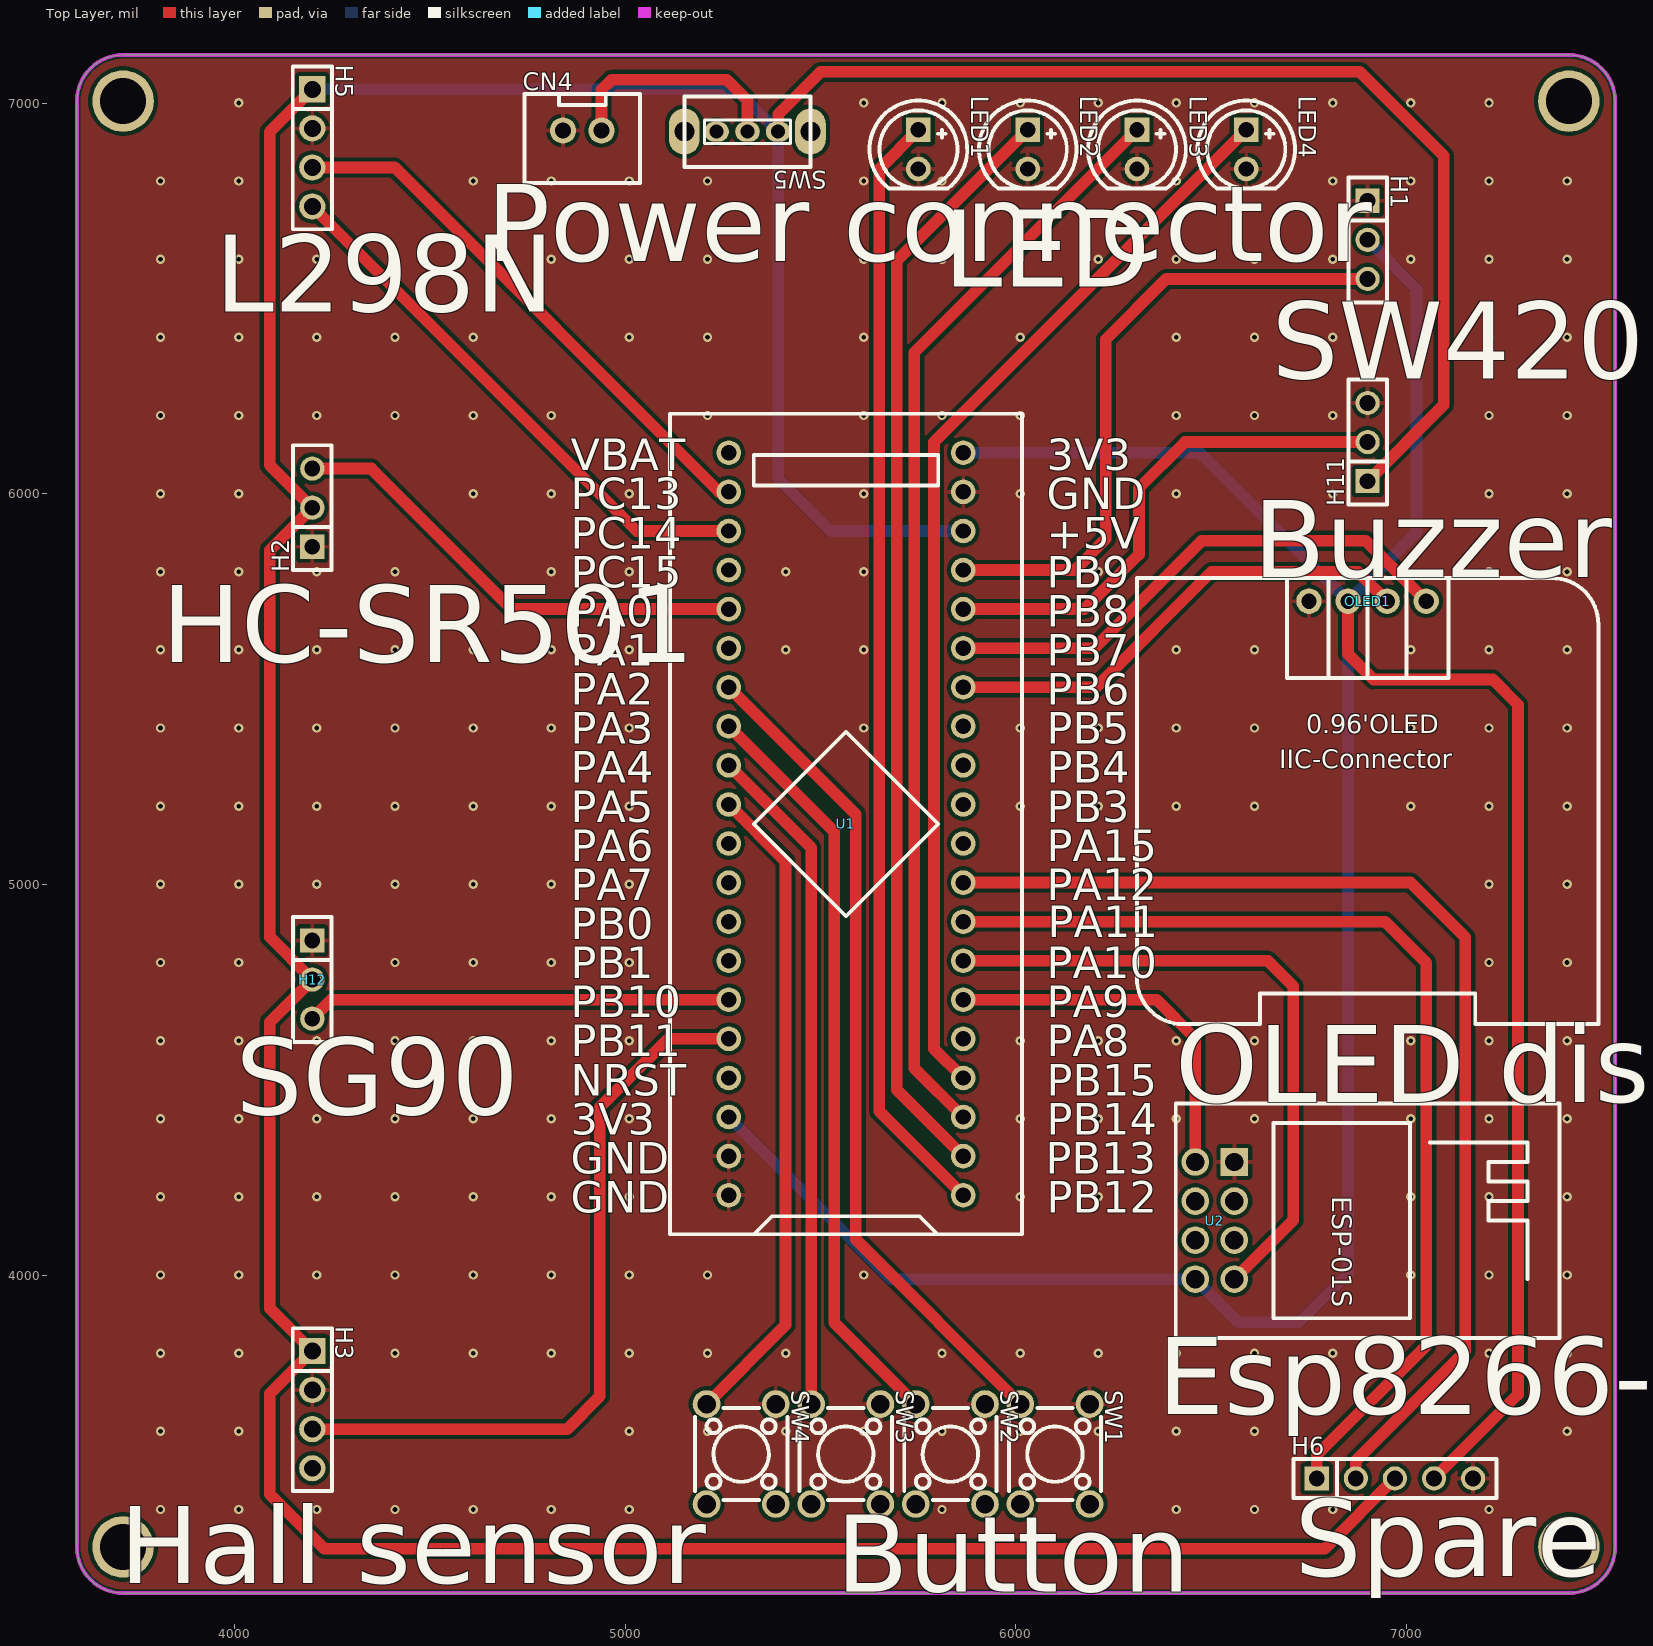
[diagram p0: Top Layer view]
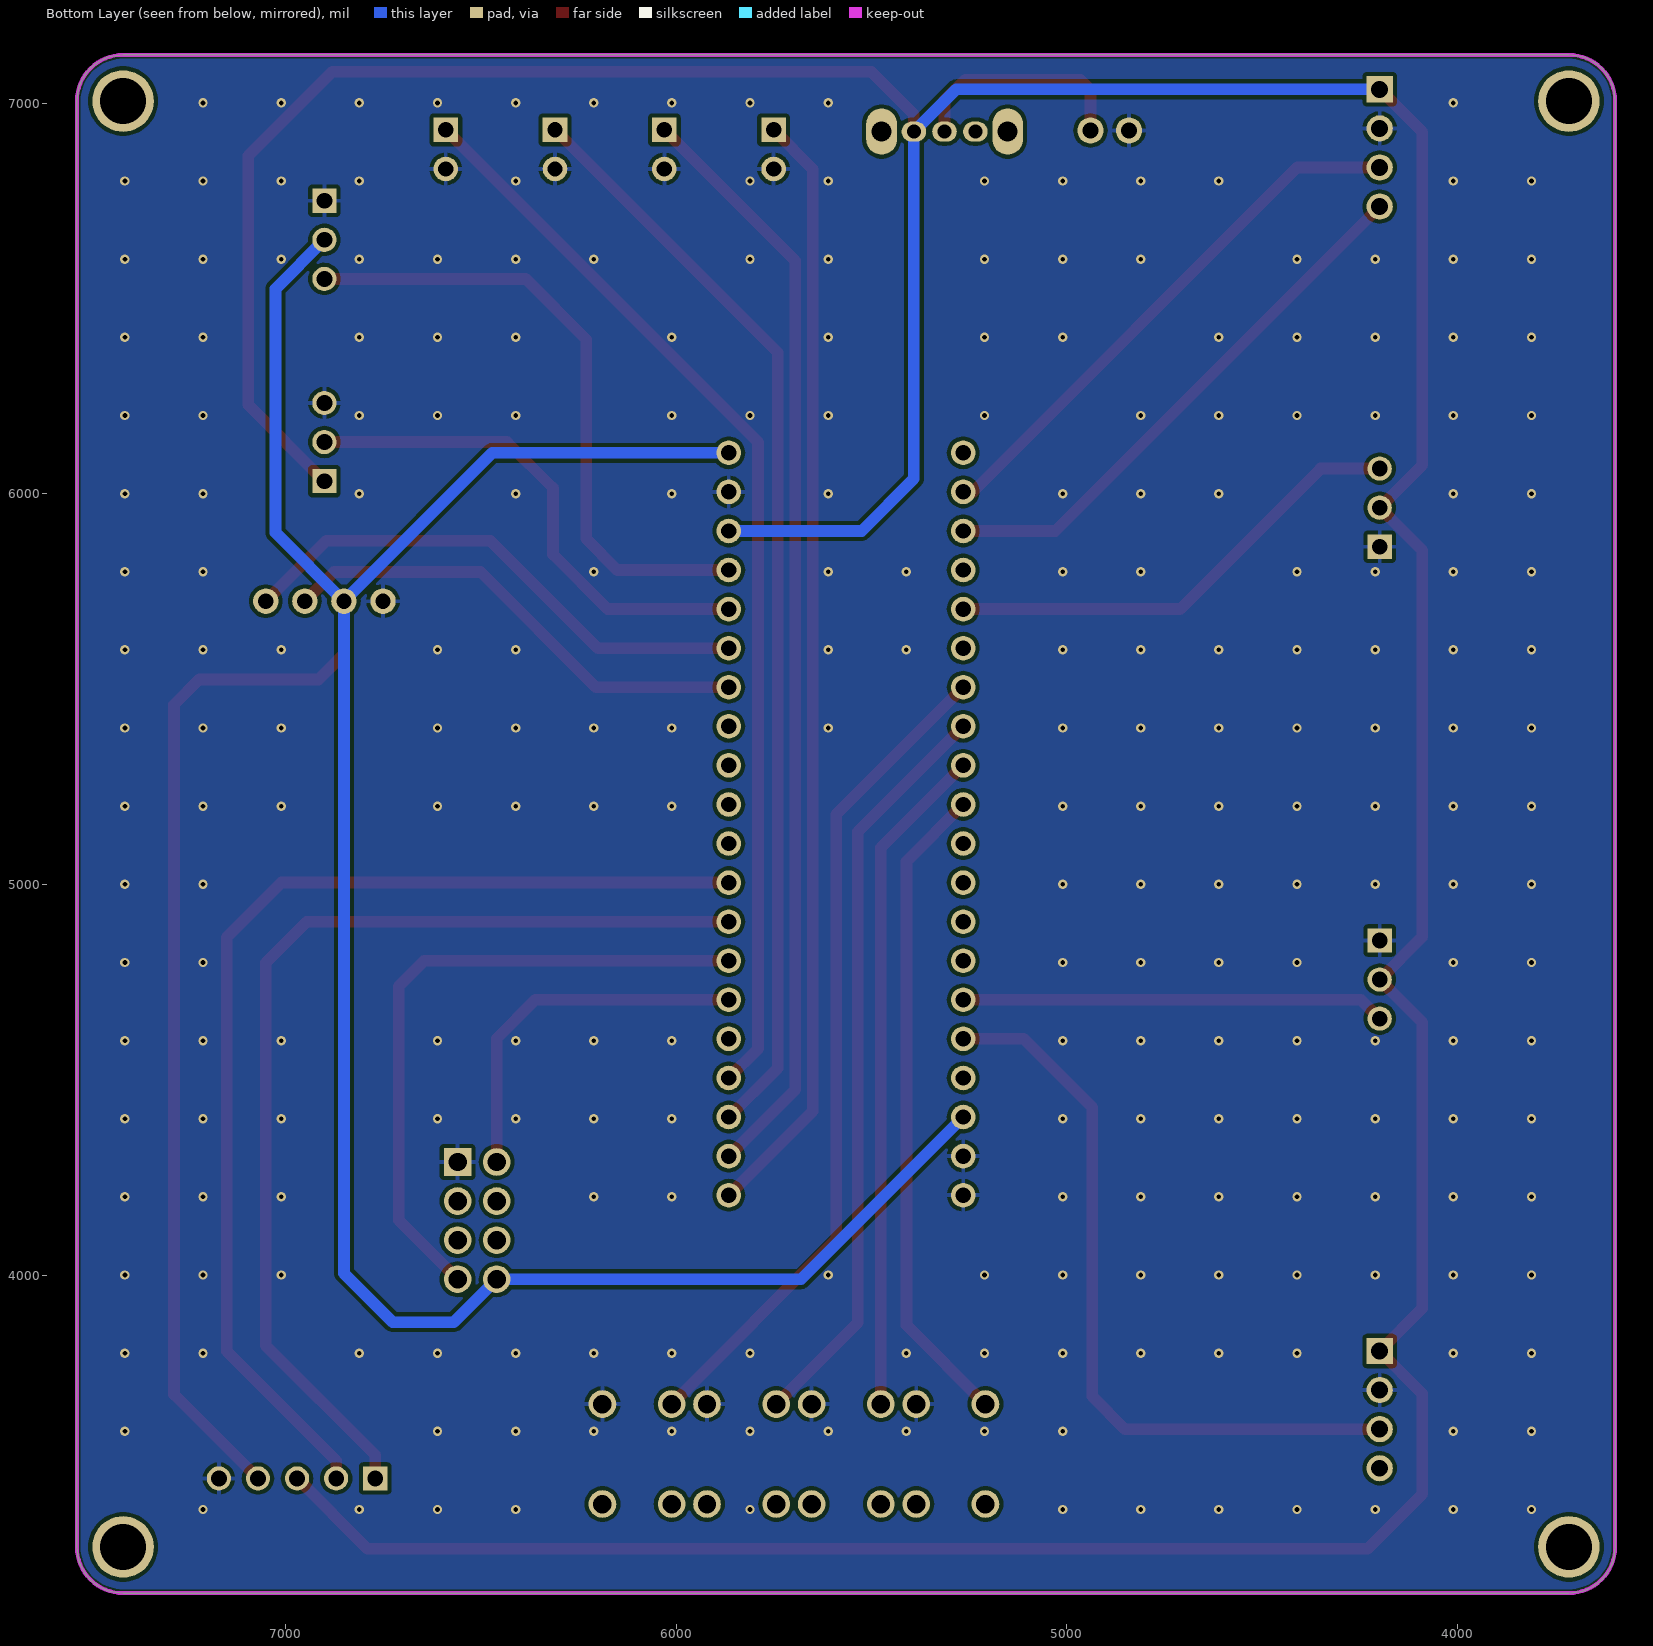
[diagram p1: Bottom Layer view, seen from below]
# Altium PCB MISC51767.pcbdoc
Units mil, origin at the board's own origin, x right, y up, seen from the top; angles counter-clockwise.
Board outline 3937.01 x 3937.01 mil, 2 copper layers (Top Layer, Bottom Layer), stack 62.206 mil thick; 20 components, 38 nets, 112 pads, 242 vias.

## Layer stack, top to bottom
Top Solder Mask Layer: solder mask 0.394, Dk 3.3
Top Layer: signal copper 1.379
Dielectric1: surface 59.449, FR4, Dk 4.5
Bottom Layer: signal copper 1.378
Bottom Solder Mask Layer: solder mask 0.394, Dk 3.3

## Board outline
3714.61,7123.5 ccw(c3714.61,7005.39) 3596.5,7005.39 3596.5,3304.61 ccw(c3714.61,3304.61) 3714.61,3186.5 7415.39,3186.5 ccw(c7415.39,3304.61) 7533.5,3304.61 7533.5,7005.39 ccw(c7415.39,7005.39) 7415.39,7123.5 3714.61,7123.5

## Design rules (kind name [scope] priority, off if disabled: settings)
BoardOutlineClearance copperThickness2oz_1 [All] p2 off: genericclearance=7.99 ignorepadtopadclearanceinfootprint=FALSE except(0: Arc-SplitContinuation Track-SplitContinuation SMDPad-SplitContinuation THPad-SplitContinuation Via-SplitContinuation Fill-SplitContinuation Region-SplitContinuation Poly-SplitContinuation Text-SplitContinuation Hole-SplitContinuation; 5.98: Arc-CutoutEdge Track-CutoutEdge SMDPad-CutoutEdge THPad-CutoutEdge Via-CutoutEdge Text-CutoutEdge; 6.9: Hole-OutlineEdge Hole-CutoutEdge; 10: Poly-OutlineEdge Poly-CutoutEdge; 11.81: Arc-OutlineEdge Track-OutlineEdge SMDPad-OutlineEdge THPad-OutlineEdge Via-OutlineEdge Fill-OutlineEdge Region-OutlineEdge Text-OutlineEdge Fill-CutoutEdge Region-CutoutEdge)
BoardOutlineClearance Plane_innerPlane_1 [All] p4 off: genericclearance=4.02 ignorepadtopadclearanceinfootprint=FALSE except(0: Arc-SplitContinuation Track-SplitContinuation SMDPad-SplitContinuation THPad-SplitContinuation Via-SplitContinuation Fill-SplitContinuation Region-SplitContinuation Poly-SplitContinuation Text-SplitContinuation Hole-SplitContinuation; 5.98: Arc-CutoutEdge Track-CutoutEdge SMDPad-CutoutEdge THPad-CutoutEdge Via-CutoutEdge Text-CutoutEdge; 6.9: Hole-OutlineEdge Hole-CutoutEdge; 10: Poly-OutlineEdge Poly-CutoutEdge; 11.81: Arc-OutlineEdge Track-OutlineEdge SMDPad-OutlineEdge THPad-OutlineEdge Via-OutlineEdge Fill-OutlineEdge Region-OutlineEdge Text-OutlineEdge Fill-CutoutEdge Region-CutoutEdge)
BoardOutlineClearance Copper_copperRegion_1 [All] p6 off: genericclearance=4.02 ignorepadtopadclearanceinfootprint=FALSE except(0: Arc-SplitContinuation Track-SplitContinuation SMDPad-SplitContinuation THPad-SplitContinuation Via-SplitContinuation Fill-SplitContinuation Region-SplitContinuation Poly-SplitContinuation Text-SplitContinuation Hole-SplitContinuation; 5.98: Arc-CutoutEdge Track-CutoutEdge SMDPad-CutoutEdge THPad-CutoutEdge Via-CutoutEdge Text-CutoutEdge; 6.9: Hole-OutlineEdge Hole-CutoutEdge; 10: Poly-OutlineEdge Poly-CutoutEdge; 11.81: Arc-OutlineEdge Track-OutlineEdge SMDPad-OutlineEdge THPad-OutlineEdge Via-OutlineEdge Fill-OutlineEdge Region-OutlineEdge Text-OutlineEdge Fill-CutoutEdge Region-CutoutEdge)
BoardOutlineClearance copperThickness1oz_1 [All] p8: genericclearance=4.02 ignorepadtopadclearanceinfootprint=FALSE except(0: Arc-SplitContinuation Track-SplitContinuation SMDPad-SplitContinuation THPad-SplitContinuation Via-SplitContinuation Fill-SplitContinuation Region-SplitContinuation Poly-SplitContinuation Text-SplitContinuation Hole-SplitContinuation; 5.98: Arc-CutoutEdge Track-CutoutEdge SMDPad-CutoutEdge THPad-CutoutEdge Via-CutoutEdge Text-CutoutEdge; 6.9: Hole-OutlineEdge Hole-CutoutEdge; 10: Poly-OutlineEdge Poly-CutoutEdge; 11.81: Arc-OutlineEdge Track-OutlineEdge SMDPad-OutlineEdge THPad-OutlineEdge Via-OutlineEdge Fill-OutlineEdge Region-OutlineEdge Text-OutlineEdge Fill-CutoutEdge Region-CutoutEdge)
Clearance copperThickness2oz [All] p1 off: gap=7.99 ignorepadtopadclearanceinfootprint=FALSE except(5.98: SMDPad-Track SMDPad-SMDPad THPad-Track SMDPad-THPad THPad-THPad Track-Via SMDPad-Via THPad-Via Via-Via Fill-SMDPad Region-SMDPad Fill-THPad Region-THPad Fill-Via Region-Via Fill-Fill Fill-Region Region-Region Arc-Track Arc-SMDPad Arc-THPad Arc-Via Fill-Arc Region-Arc Arc-Arc Text-Track SMDPad-Text Text-THPad Text-Via Fill-Text Region-Text Arc-Text Text-Text; 6.9: Hole-Track Hole-SMDPad Hole-THPad Hole-Via Fill-Hole Region-Hole Hole-Arc Hole-Text; 10: Poly-Track Poly-SMDPad Poly-THPad Poly-Via Poly-Fill Poly-Region Poly-Poly Poly-Arc Poly-Text Poly-Hole; 11.81: Fill-Track Region-Track)
Clearance Plane_innerPlane [All] p3 off: gap=4.02 ignorepadtopadclearanceinfootprint=FALSE except(5.98: SMDPad-Track SMDPad-SMDPad THPad-Track SMDPad-THPad THPad-THPad Track-Via SMDPad-Via THPad-Via Via-Via Fill-SMDPad Region-SMDPad Fill-THPad Region-THPad Fill-Via Region-Via Fill-Fill Fill-Region Region-Region Arc-Track Arc-SMDPad Arc-THPad Arc-Via Fill-Arc Region-Arc Arc-Arc Text-Track SMDPad-Text Text-THPad Text-Via Fill-Text Region-Text Arc-Text Text-Text; 6.9: Hole-Track Hole-SMDPad Hole-THPad Hole-Via Fill-Hole Region-Hole Hole-Arc Hole-Text; 10: Poly-Track Poly-SMDPad Poly-THPad Poly-Via Poly-Fill Poly-Region Poly-Poly Poly-Arc Poly-Text Poly-Hole; 11.81: Fill-Track Region-Track)
Clearance Copper_copperRegion [All] p5 off: gap=4.02 ignorepadtopadclearanceinfootprint=FALSE except(5.98: SMDPad-Track SMDPad-SMDPad THPad-Track SMDPad-THPad THPad-THPad Track-Via SMDPad-Via THPad-Via Via-Via Fill-SMDPad Region-SMDPad Fill-THPad Region-THPad Fill-Via Region-Via Fill-Fill Fill-Region Region-Region Arc-Track Arc-SMDPad Arc-THPad Arc-Via Fill-Arc Region-Arc Arc-Arc Text-Track SMDPad-Text Text-THPad Text-Via Fill-Text Region-Text Arc-Text Text-Text; 6.9: Hole-Track Hole-SMDPad Hole-THPad Hole-Via Fill-Hole Region-Hole Hole-Arc Hole-Text; 10: Poly-Track Poly-SMDPad Poly-THPad Poly-Via Poly-Fill Poly-Region Poly-Poly Poly-Arc Poly-Text Poly-Hole; 11.81: Fill-Track Region-Track)
Clearance copperThickness1oz [All] p7: gap=4.02 ignorepadtopadclearanceinfootprint=FALSE except(5.98: SMDPad-Track SMDPad-SMDPad THPad-Track SMDPad-THPad THPad-THPad Track-Via SMDPad-Via THPad-Via Via-Via Fill-SMDPad Region-SMDPad Fill-THPad Region-THPad Fill-Via Region-Via Fill-Fill Fill-Region Region-Region Arc-Track Arc-SMDPad Arc-THPad Arc-Via Fill-Arc Region-Arc Arc-Arc Text-Track SMDPad-Text Text-THPad Text-Via Fill-Text Region-Text Arc-Text Text-Text; 6.9: Hole-Track Hole-SMDPad Hole-THPad Hole-Via Fill-Hole Region-Hole Hole-Arc Hole-Text; 10: Poly-Track Poly-SMDPad Poly-THPad Poly-Via Poly-Fill Poly-Region Poly-Poly Poly-Arc Poly-Text Poly-Hole; 11.81: Fill-Track Region-Track)
DiffPairsRouting differentialPair [All] p1: maxlimit=6 minlimit=6 mostfreqgap=6 toplayer_minwidth=5 toplayer_prefwidth=10 toplayer_maxwidth=100 toplayer_mingap=6 toplayer_prefgap=6 toplayer_maxgap=6 bottomlayer_minwidth=5 bottomlayer_prefwidth=10 bottomlayer_maxwidth=100 bottomlayer_mingap=6 bottomlayer_prefgap=6 bottomlayer_maxgap=6 maxuncoupledlength=10
HoleToHoleClearance otherClearance [All] p1: gap=11.81 allowstackedmicrovias=TRUE
Length netLength [All] p1: minlimit=0 maxlimit=0
PasteMaskExpansion pasteMaskExpansion [All] p1: expansion=0
PlaneConnect innerPlane [All] p1: planeconnectstyle=Relief reliefexpansion=20 reliefentries=4 reliefconductorwidth=10 reliefairgap=10
PolygonConnect copperRegion [All] p1: connectstyle=Relief reliefconductorwidth=10 reliefentries=4 polygonreliefangle="90 Angle" airgapwidth=10 via.connectstyle=Relief via.reliefconductorwidth=10 via.reliefentries=4 via.polygonreliefangle="90 Angle" via.airgapwidth=10
RoutingVias viaSize [All] p1: holewidth=12.01 width=24.02 viastyle="Through Hole" minholewidth=11.81 minwidth=19.68 maxholewidth=248.03 maxwidth=393.7
SolderMaskExpansion solderMaskExpansion [IsVia] p1: expansion=-1000 istentingtop=TRUE
SolderMaskExpansion solderMaskExpansion [All] p2: expansion=2 istentingtop=FALSE
Width copperThickness2oz_2 [All] p1 off: maxlimit=100 minlimit=8 preferedwidth=10
Width copperThickness1oz_2 [All] p2: maxlimit=100 minlimit=5 preferedwidth=10

## Components (designator, comment, footprint, x,y, rotation, side; value= is the part's Value field where it differs from the comment)
CN4 "XH2.54*2P_through-hole" CONN-TH_2P-P2.50-XH2.54-2P 4890,6930 r0 top
H1 "" HDR-TH_3P-P2.54-V-F 6900,6650.1 r270 top
H2 "" HDR-TH_3P-P2.54-V-F 4199,5964.65 r90 top
H3 "" HDR-TH_4P-P2.54-V-F 4199,3656.13 r270 top
H5 "" HDR-TH_4P-P2.54-V-F 4199,6885.41 r270 top
H6 "" HDR-TH_5P-P2.54-V-F 6970,3480 r0 top
H11 "" HDR-TH_3P-P2.54-V-F 6900,6132.57 r90 top
H12 "" HDR-TH_3P-P2.54-V-F 4199,4756.89 r270 top
LED1 "" LED-TH_5mm 5750.35,6881.55 r270 top
LED2 "" LED-TH_5mm 6030.04,6881.55 r270 top
LED3 "" LED-TH_5mm 6309.72,6881.55 r270 top
LED4 "" LED-TH_5mm 6589.41,6881.55 r270 top
OLED1 "" 0.96OLED_4P 6900,5725.27 r0 top
SW1 "" SW-TH_4P-L6.0-W6.0-P4.50-LS6.5 6099.85,3542.47 r270 top
SW2 "" SW-TH_4P-L6.0-W6.0-P4.50-LS6.5 5832.14,3542.47 r270 top
SW3 "" SW-TH_4P-L6.0-W6.0-P4.50-LS6.5 5564.43,3542.47 r270 top
SW4 "" SW-TH_4P-L6.0-W6.0-P4.50-LS6.5 5296.72,3542.47 r270 top
SW5 "" 拨动开关 5317.9,6927.05 r180 top
U1 "STM32F103C8T6-Card" CONN-TH_L53.3-W22.9_STM32F103C8T6-CARD 5565,5155 r90 top
U2 "ESP-01S" WIFIM-TH_ESP-01S 6509,4139.91 r270 top

## Footprints (in the part's own frame and the unit in brackets; to place one, negate y for a bottom-side part, rotate by r counter-clockwise, add the part's x,y. Pads: shape width x height; smd on the part's side, far side on the other; paste and mask are expansions set on the pad)
0.96OLED_4P [mm]
  round 1.65 hole 1 copper offset 0,0: 1(-3.81,-0.001) 2(-1.27,0.002) 3(1.27,0.002) 4(3.81,0.002)
  silkscreen extent -15,-27.5 15,1.5
CONN-TH_2P-P2.50-XH2.54-2P [mm]
  round 1.7 hole 1.05 paste+0 mask+0.05: 1(1.25,0) 2(-1.25,0)
  silkscreen extent -3.75,-3.42 3.75,2.37
CONN-TH_L53.3-W22.9_STM32F103C8T6-CARD [mm]
  round 1.6 hole 1: 1(-24.13,-7.62) 2(-21.59,-7.62) 3(-19.05,-7.62) 4(-16.51,-7.62) 5(-13.97,-7.62) 6(-11.43,-7.62) 7(-8.89,-7.62) 8(-6.35,-7.62) 9(-3.81,-7.62) 10(-1.27,-7.62) 11(1.27,-7.62) 12(3.81,-7.62) 13(6.35,-7.62) 14(8.89,-7.62) 15(11.43,-7.62) 16(13.97,-7.62) 17(16.51,-7.62) 18(19.05,-7.62) 19(21.59,-7.62) 20(24.13,-7.62) 21(24.13,7.62) 22(21.59,7.62) 23(19.05,7.62) 24(16.51,7.62) 25(13.97,7.62) 26(11.43,7.62) 27(8.89,7.62) 28(6.35,7.62) 29(3.81,7.62) 30(1.27,7.62) 31(-1.27,7.62) 32(-3.81,7.62) 33(-6.35,7.62) 34(-8.89,7.62) 35(-11.43,7.62) 36(-13.97,7.62) 37(-16.51,7.62) 38(-19.05,7.62) 39(-21.59,7.62) 40(-24.13,7.62)
  silkscreen extent -26.67,-11.43 26.67,11.43
HDR-TH_3P-P2.54-V-F [mil]
  rect 62x62 hole 40.16: 1(-100,0)
  round 62 hole 40.16: 2(0,0) 3(100,0)
  silkscreen extent -160,-49 160,49
HDR-TH_4P-P2.54-V-F [mm]
  rect 1.7x1.7 hole 1.1: 1(-3.81,0)
  round 1.7 hole 1.1: 2(-1.27,0) 3(1.27,0) 4(3.81,0)
  silkscreen extent -5.29,-1.27 5.29,1.27
HDR-TH_5P-P2.54-V-F [mil]
  rect 62x62 hole 40.16: 1(-200,0)
  round 62 hole 40.16: 2(-100,0) 3(0,0) 4(100,0) 5(200,0)
  silkscreen extent -260,-50 260,50
LED-TH_5mm [mm]
  rect 1.6x1.6 hole 1 paste+0 mask+0.051: 1(-1.27,0)
  round 1.6 hole 1 paste+0 mask+0.051: 2(1.27,0)
  silkscreen extent -3.17,-3.17 2.54,3.17
SW-TH_4P-L6.0-W6.0-P4.50-LS6.5 [mm]
  round 1.8 hole 1.2: 1(-3.25,2.25) 2(3.25,2.25) 3(-3.25,-2.25) 4(3.25,-2.25)
  silkscreen extent -3,-3 3,3
WIFIM-TH_ESP-01S [mm]
  rect 1.8x1.8 hole 1.2: 1(-3.81,1.27)
  round 1.8 hole 1.2: 2(-1.27,1.27) 3(1.27,1.27) 4(3.81,1.27) 5(3.81,-1.27) 6(1.27,-1.27) 7(-1.27,-1.27) 8(-3.81,-1.27)
  silkscreen extent -7.62,-2.54 7.62,22.4
拨动开关 [mil]
  oval 63x51.2 hole 35.4 paste+0 mask+2: 1(-73.4,0) 2(5,0) 3(84,0)
  oval 78.7x118.1 hole 51.2 paste+0 mask+2: 4(166.7,0) 5(-156.1,0)
  silkscreen extent -156,-90 167,90

## Free pads (board coordinates)
  round 157.48 hole 118.11: 1(3714.61,7005.39) 1(3714.61,3304.61) 1(7415.39,7005.39) 1(7415.39,3304.61)

## Via types
v1: diameter 24.02, hole 12, Top Layer to Bottom Layer, 242 vias

## Nets (pads, with @x,y where several pads share a name; then routed paths per layer and width w, separated by ;. In a path a pad name is that pad's centre, name@x,y a point inside that pad or via, vN(x,y) a via of type N, cw(c..) or ccw(c..) an arc to the next point about the centre after c; other vN are vias at no path point)
$1N17118: CN4.1 SW5.2 | length 590.5
  Top Layer w30: CN4.1 4939.22,7034.22 4965,7060 5260,7060 5312.9,7007.1 SW5.2
+5V: H2.2 H3.1 H5.1 H6.3 H11.1 H12.2 SW5.1 U1.18 | length 12373.9
  Top Layer w30: H5.1 4090,6926.41 4090,6073.65 H2.2 4090,5855.65 4090,4865.89 H12.2 4090,4647.89 4090,3915.13 H3.1 4090,3697.13 4090,3440 4230,3300 6790,3300 H6.3 ; SW5.1 5391.3,6971.3 5500,7080 6880,7080 7095,6865 7095,6227.57 H11.1
  Bottom Layer w30: H5.1 5282.93,7035.41 SW5.1 5391.3,6038.7 5525,5905 U1.18
GND: CN4.2 H1.1 H2.1 H3.2 H5.2 H6.5 H11.3 H12.1 LED1.2 LED2.2 LED3.2 LED4.2 OLED1.1 SW1.1 SW2.1 SW3.1 SW4.1 U1.19 U1.39 U1.40 U2.1
  other v1: 3810.6,3400.6 4010.6,3400.6 4210.6,3400.6 4410.6,3400.6 4610.6,3400.6 4810.6,3400.6 5010.6,3400.6 5810.6,3400.6 6410.6,3400.6 6610.6,3400.6 6810.6,3400.6 7210.6,3400.6 3810.6,3600.6 4010.6,3600.6 5010.6,3600.6 5210.6,3600.6 5410.6,3600.6 5610.6,3600.6 5810.6,3600.6 6010.6,3600.6 6210.6,3600.6 6410.6,3600.6 6610.6,3600.6 7410.6,3600.6 3810.6,3800.6 4010.6,3800.6 4410.6,3800.6 4610.6,3800.6 4810.6,3800.6 5010.6,3800.6 5210.6,3800.6 5410.6,3800.6 5810.6,3800.6 6010.6,3800.6 6210.6,3800.6 6410.6,3800.6 6610.6,3800.6 6810.6,3800.6 7210.6,3800.6 7410.6,3800.6 3810.6,4000.6 4010.6,4000.6 4210.6,4000.6 4410.6,4000.6 4610.6,4000.6 4810.6,4000.6 5010.6,4000.6 5210.6,4000.6 5610.6,4000.6 7010.6,4000.6 7210.6,4000.6 7410.6,4000.6 3810.6,4200.6 4010.6,4200.6 4210.6,4200.6 4410.6,4200.6 4610.6,4200.6 4810.6,4200.6 5010.6,4200.6 6010.6,4200.6 6210.6,4200.6 7010.6,4200.6 7210.6,4200.6 7410.6,4200.6 3810.6,4400.6 4010.6,4400.6 4210.6,4400.6 4410.6,4400.6 4610.6,4400.6 4810.6,4400.6 5010.6,4400.6 6010.6,4400.6 6210.6,4400.6 6410.6,4400.6 6610.6,4400.6 7010.6,4400.6 7210.6,4400.6 7410.6,4400.6 3810.6,4600.6 4010.6,4600.6 4210.6,4600.6 4410.6,4600.6 4610.6,4600.6 4810.6,4600.6 5010.6,4600.6 6010.6,4600.6 6210.6,4600.6 6410.6,4600.6 6610.6,4600.6 7010.6,4600.6 7210.6,4600.6 7410.6,4600.6 3810.6,4800.6 4010.6,4800.6 4410.6,4800.6 4610.6,4800.6 4810.6,4800.6 5010.6,4800.6 7210.6,4800.6 7410.6,4800.6 3810.6,5000.6 4010.6,5000.6 4210.6,5000.6 4410.6,5000.6 4610.6,5000.6 4810.6,5000.6 5010.6,5000.6 7210.6,5000.6 7410.6,5000.6 3810.6,5200.6 4010.6,5200.6 4210.6,5200.6 4410.6,5200.6 4610.6,5200.6 4810.6,5200.6 5010.6,5200.6 6010.6,5200.6 6210.6,5200.6 6410.6,5200.6 6610.6,5200.6 7010.6,5200.6 7210.6,5200.6 7410.6,5200.6 3810.6,5400.6 4010.6,5400.6 4210.6,5400.6 4410.6,5400.6 4610.6,5400.6 4810.6,5400.6 5010.6,5400.6 5610.6,5400.6 6010.6,5400.6 6210.6,5400.6 6410.6,5400.6 6610.6,5400.6 7010.6,5400.6 7210.6,5400.6 7410.6,5400.6 3810.6,5600.6 4010.6,5600.6 4210.6,5600.6 4410.6,5600.6 4610.6,5600.6 4810.6,5600.6 5010.6,5600.6 5410.6,5600.6 5610.6,5600.6 6410.6,5600.6 6610.6,5600.6 7010.6,5600.6 7210.6,5600.6 7410.6,5600.6 3810.6,5800.6 4010.6,5800.6 4210.6,5800.6 4410.6,5800.6 4810.6,5800.6 5010.6,5800.6 5410.6,5800.6 5610.6,5800.6 6210.6,5800.6 7210.6,5800.6 7410.6,5800.6 3810.6,6000.6 4010.6,6000.6 4610.6,6000.6 4810.6,6000.6 5010.6,6000.6 5610.6,6000.6 6010.6,6000.6 6410.6,6000.6 6810.6,6000.6 7210.6,6000.6 7410.6,6000.6 3810.6,6200.6 4010.6,6200.6 4210.6,6200.6 4410.6,6200.6 4610.6,6200.6 4810.6,6200.6 5210.6,6200.6 5610.6,6200.6 5810.6,6200.6 6010.6,6200.6 6410.6,6200.6 6610.6,6200.6 6810.6,6200.6 7210.6,6200.6 7410.6,6200.6 3810.6,6400.6 4010.6,6400.6 4210.6,6400.6 4410.6,6400.6 4610.6,6400.6 5010.6,6400.6 5210.6,6400.6 5610.6,6400.6 6010.6,6400.6 6410.6,6400.6 6610.6,6400.6 6810.6,6400.6 7210.6,6400.6 7410.6,6400.6 3810.6,6600.6 4010.6,6600.6 4210.6,6600.6 4410.6,6600.6 4810.6,6600.6 5010.6,6600.6 5210.6,6600.6 5610.6,6600.6 5810.6,6600.6 6210.6,6600.6 6410.6,6600.6 6610.6,6600.6 6810.6,6600.6 7010.6,6600.6 7210.6,6600.6 7410.6,6600.6 3810.6,6800.6 4010.6,6800.6 4610.6,6800.6 4810.6,6800.6 5010.6,6800.6 5210.6,6800.6 5610.6,6800.6 5810.6,6800.6 6410.6,6800.6 6810.6,6800.6 7010.6,6800.6 7210.6,6800.6 7410.6,6800.6 4010.6,7000.6 5610.6,7000.6 5810.6,7000.6 6010.6,7000.6 6210.6,7000.6 6410.6,7000.6 6610.6,7000.6 6810.6,7000.6 7010.6,7000.6 7210.6,7000.6
NRST: U1.37
PA0: H2.3 U1.25 | length 1215
  Top Layer w30: H2.3 4350.35,6064.65 4710,5705 U1.25
PA1: U1.26
PA2: SW1.3 U1.27 | length 2143.7
  Top Layer w30: U1.27 5590,5180 5590,4091.69 SW1.3
PA3: SW2.3 U1.28 | length 1932.8
  Top Layer w30: U1.28 5535,5135 5535,3878.98 SW2.3
PA4: SW3.3 U1.29 | length 1721.9
  Top Layer w30: U1.29 5475.85,5094.15 SW3.3
PA5: SW4.3 U1.30 | length 1678.3
  Top Layer w30: SW4.3 5410,3872.28 5410,5060 U1.30
PA6: U1.31
PA7: U1.32
PA8: U1.5
PA9: U1.6 U2.8 | length 951.1
  Top Layer w30: U1.6 6360,4705 6459,4606 U2.8
PA10: U1.7 U2.4 | length 1684.6
  Top Layer w30: U1.7 6645,4805 6710,4740 6710,4140.91 U2.4
PA11: H6.1 U1.8 | length 2664.5
  Top Layer w30: U1.8 6945,4905 7050,4800 7050,3820 6770,3540 H6.1
PA12: H6.2 U1.9 | length 2844
  Top Layer w30: U1.9 7010,5005 7150,4865 7150,3805.6 6870,3525.6 H6.2
PA15: U1.10
PB0: U1.33
PB1: U1.34
PB3: U1.11
PB4: U1.12
PB5: U1.13
PB6: OLED1.3 U1.14 | length 1238.1
  Top Layer w30: U1.14 6205,5505 6500,5800 6875.32,5800 OLED1.3
PB7: OLED1.4 U1.15 | length 1363
  Top Layer w30: U1.15 6200,5605 6475,5880 6895.32,5880 OLED1.4
PB8: H11.2 U1.16 | length 1311.7
  Top Layer w30: U1.16 6175,5705 6315,5845 6315,6015 6432.57,6132.57 H11.2
PB9: H1.3 U1.17 | length 1642.4
  Top Layer w30: U1.17 6150,5805 6230,5885 6230,6395 6385.1,6550.1 H1.3
PB10: H12.3 U1.35 | length 1085.9
  Top Layer w30: H12.3 4247.11,4705 U1.35
PB11: H3.3 U1.36 | length 1913.2
  Top Layer w30: H3.3 4851.13,3606.13 4935,3690 4935,4430 5110,4605 U1.36
PB12: LED1.1 U1.1 | length 2857.2
  Top Layer w30: LED1.1 5650,6831.2 5650,4420 U1.1
PB13: LED2.1 U1.2 | length 2835.7
  Top Layer w30: U1.2 5695,4475 5695,6596.52 LED2.1
PB14: LED3.1 U1.3 | length 2814.3
  Top Layer w30: U1.3 5740,4530 5740,6361.83 LED3.1
PB15: LED4.1 U1.4 | length 2788.7
  Top Layer w30: U1.4 5790,4580 5790,6132.15 LED4.1
PC13: H5.3 U1.22 | length 1410
  Top Layer w30: H5.3 4409.59,6835.41 5240,6005 U1.22
PC14: H5.4 U1.23 | length 1410
  Top Layer w30: H5.4 5029.41,5905 U1.23
PC15: U1.24
VBAT: U1.21
VCC: H1.2 H6.4 OLED1.2 U1.20 U1.38 U2.5 | length 8459.1
  Top Layer w30: OLED1.2 6850,5590 6915,5525 7220,5525 7285,5460 7285,3695 H6.4
  Bottom Layer w30: U1.38 5680.09,3989.91 U2.5 6568.9,3880 6725,3880 6850,4005 OLED1.2 ; U1.20 6470.32,6105 OLED1.2 ; H1.2 7025,6525.1 7025,5900.32 OLED1.2
pads on no net: H3.4 SW1.2 SW1.4 SW2.2 SW2.4 SW3.2 SW3.4 SW4.2 SW4.4 SW5.3 SW5.4 SW5.5 U2.2 U2.3 U2.6 U2.7

## Polygon pours and split planes (outlines as drawn)
GND on Bottom Layer (solid, remove dead copper, pour order 2): 3525,7245 3525,3080 7700,3080 7700,7245
GND on Top Layer (solid, remove dead copper, pour order 2): 3000,7415 3000,3000 7930,3000 7930,7415

## Keep-outs
Board Outline Layer:
  the board outline again, w10

## Silkscreen, mask and mechanical layers (free items; w line width, h text height)
Top Silkscreen Layer:
  text "Power connector" at 4645,6595 h196.85
  text "LED" at 5815,6530 h196.85
  text "L298N" at 3950.85,6465.86 h196.85
  text "SW420" at 6654.68,6294.7 h196.85
  text "VBAT" at 4860.95,6060 h80
  text "3V3" at 6079.16,6060 h80
  text "PC13" at 4860.95,5960 h80
  text "GND" at 6079.16,5960 h80
  text "PC14" at 4860.95,5860 h80
  text "+5V" at 6079.16,5860 h80
  text "Buzzer" at 6606.81,5786.71 h196.85
  text "PC15" at 4860.95,5760 h80
  text "PB9" at 6079.16,5760 h80
  text "PA0" at 4860.95,5660 h80
  text "PB8" at 6079.16,5660 h80
  text "HC-SR501" at 3813.95,5568.53 h196.85
  text "PA1" at 4860.95,5560 h80
  text "PB7" at 6079.16,5560 h80
  text "PA2" at 4860.95,5460 h80
  text "PB6" at 6079.16,5460 h80
  text "PA3" at 4860.95,5360 h80
  text "PB5" at 6079.16,5360 h80
  text "PA4" at 4860.95,5260 h80
  text "PB4" at 6079.16,5260 h80
  text "PA5" at 4860.95,5160 h80
  text "PB3" at 6079.16,5160 h80
  text "PA6" at 4860.95,5060 h80
  text "PA15" at 6079.16,5060 h80
  text "PA7" at 4860.95,4960 h80
  text "PA12" at 6079.16,4960 h80
  text "PA11" at 6080.95,4865 h80
  text "PB0" at 4860.95,4860 h80
  text "PB1" at 4860.95,4760 h80
  text "PA10" at 6079.16,4760 h80
  text "PB10" at 4860.95,4660 h80
  text "PA9" at 6079.16,4660 h80
  text "PB11" at 4860.95,4560 h80
  text "PA8" at 6079.16,4560 h80
  text "NRST" at 4860.95,4460 h80
  text "PB15" at 6079.16,4460 h80
  text "OLED display" at 6408.02,4442.89 h196.85
  text "SG90" at 4002.9,4410.76 h196.85
  text "3V3" at 4860.95,4360 h80
  text "PB14" at 6079.16,4360 h80
  text "GND" at 4860.95,4260 h80
  text "PB13" at 6075.95,4260 h80
  text "GND" at 4860.95,4160 h80
  text "PB12" at 6079.16,4160 h80
  text "Esp8266-01s" at 6363.13,3643.65 h196.85
  text "Spare" at 6714.18,3230 h196.85
  text "Hall sensor" at 3706.13,3211.57 h196.85
  text "Button" at 5540,3190 h196.85